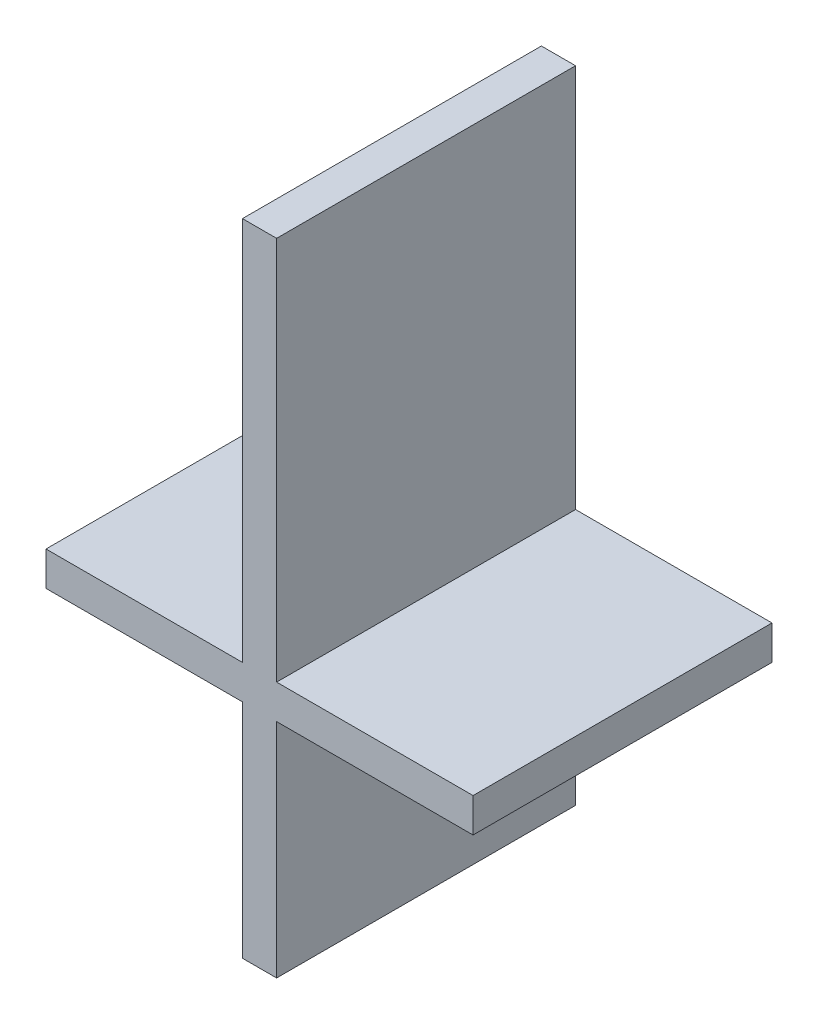
SolidWorks part; units mm, degrees
ref_plane "Front Plane" through (0, 0, 0) normal (0, 0, 1) x (1, 0, 0)
ref_plane "Top Plane" through (0, 0, 0) normal (0, 1, 0) x (1, 0, 0)
ref_plane "Right Plane" through (0, 0, 0) normal (1, 0, 0) x (0, 0, -1)
sketch "Sketch1" plane through (0, 0, 0) normal (0, 0, 1) x (1, 0, 0)
  line L0 (4, -4) -> (4, -56)
  line L1 (50, 4) -> (4, 4)
  line L2 (50, 4) -> (50, -4)
  line L3 (50, -4) -> (4, -4)
  line L4 (-50, 4) -> (-50, -4)
  line L5 (50, 4) -> (-50, -4) construction
  line L6 (50, -4) -> (-50, 4) construction
  line L11 (4, 94) -> (-4, 94)
  line L12 (4, 94) -> (4, 4)
  line L13 (4, -56) -> (-4, -56)
  line L14 (-4, 94) -> (-4, 4)
  line L15 (4, 94) -> (-4, -56) construction
  line L16 (4, -56) -> (-4, 94) construction
  line L17 (-4, 4) -> (-50, 4)
  line L19 (-4, -4) -> (-50, -4)
  line L20 (-4, -4) -> (-4, -56)
  point P0 (0, 0)
  point P6 (0, 0)
  point P7 (0, 19)
  dimension "D1" = 150
  dimension "D2" = 90
  dimension "D3" = 8
  dimension "D4" = 8
  dimension "D5" = 100
extrude "Boss-Extrude1" add sketch "Sketch1" along normal blind 70
